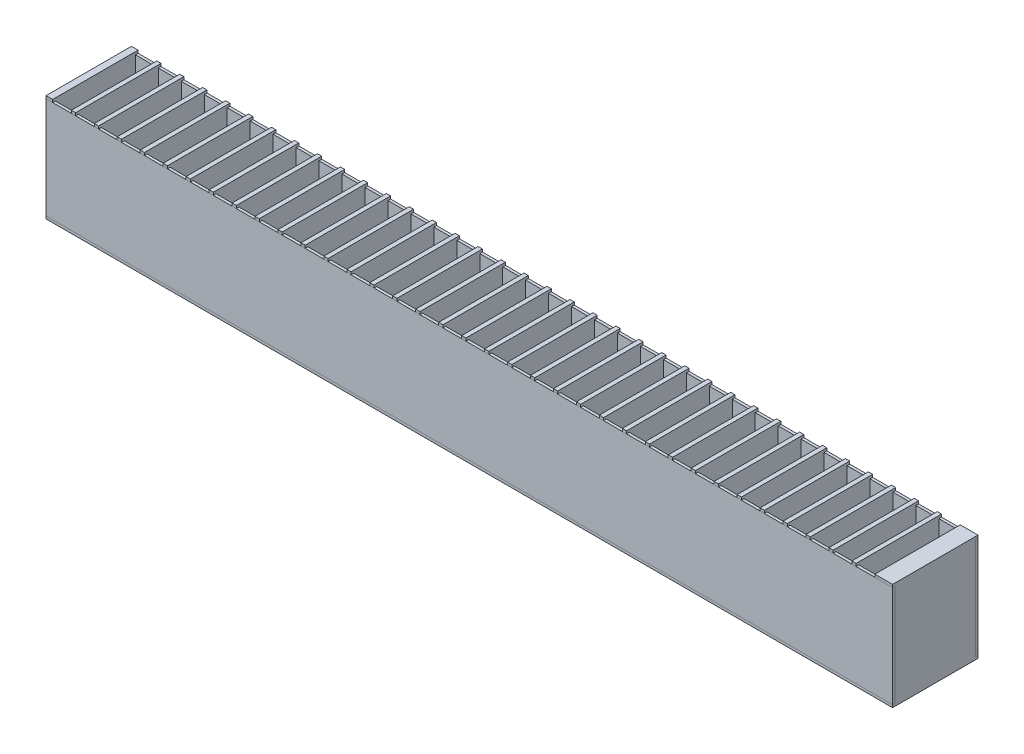
SolidWorks part; units mm, degrees
ref_plane "Front Plane" through (0, 0, 0) normal (0, 0, 1) x (1, 0, 0)
ref_plane "Top Plane" through (0, 0, 0) normal (0, 1, 0) x (1, 0, 0)
ref_plane "Right Plane" through (0, 0, 0) normal (1, 0, 0) x (0, 0, -1)
other "Configuration Table"
sketch "Sketch1" plane through (0, 0, 0) normal (0, 1, 0) x (1, 0, 0)
  line L0 (-0.4, -6) -> (-3.9, -6)
  line L1 (-78.2442, 8) -> (80.3234, 8)
  line L2 (-78.2442, 8) -> (-78.2442, -8)
  line L3 (-78.2442, -8) -> (80.3234, -8)
  line L4 (80.3234, 8) -> (80.3234, -8)
  line L5 (-55, 0) -> (55, 0) construction
  line L6 (0, -55) -> (0, 55) construction
  line L7 (-0.4, 1) -> (-3.9, 1)
  line L8 (-0.4, 1) -> (-0.4, 6)
  line L9 (-0.4, 6) -> (-3.9, 6)
  line L10 (-3.9, 1) -> (-3.9, 6)
  line L11 (-3.9, -1) -> (-3.9, -6)
  line L12 (-0.4, -1) -> (-3.9, -1)
  line L13 (-0.4, -1) -> (-0.4, -6)
  line L14 (3.9, 1) -> (3.9, 6)
  line L15 (3.9, 1) -> (0.4, 1)
  line L16 (0.4, 1) -> (0.4, 6)
  line L17 (3.9, 6) -> (0.4, 6)
  line L18 (3.9, -6) -> (0.4, -6)
  line L19 (0.4, -1) -> (0.4, -6)
  line L20 (3.9, -1) -> (0.4, -1)
  line L21 (3.9, -1) -> (3.9, -6)
  line L22 (8.2, 1) -> (8.2, 6)
  line L23 (8.2, 1) -> (4.7, 1)
  line L24 (4.7, 1) -> (4.7, 6)
  line L25 (8.2, 6) -> (4.7, 6)
  line L26 (8.2, -6) -> (4.7, -6)
  line L27 (4.7, -1) -> (4.7, -6)
  line L28 (8.2, -1) -> (4.7, -1)
  line L29 (8.2, -1) -> (8.2, -6)
  line L30 (12.5, 1) -> (12.5, 6)
  line L31 (12.5, 1) -> (9, 1)
  line L32 (9, 1) -> (9, 6)
  line L33 (12.5, 6) -> (9, 6)
  line L34 (12.5, -6) -> (9, -6)
  line L35 (9, -1) -> (9, -6)
  line L36 (12.5, -1) -> (9, -1)
  line L37 (12.5, -1) -> (12.5, -6)
  line L38 (16.8, 1) -> (16.8, 6)
  line L39 (16.8, 1) -> (13.3, 1)
  line L40 (13.3, 1) -> (13.3, 6)
  line L41 (16.8, 6) -> (13.3, 6)
  line L42 (16.8, -6) -> (13.3, -6)
  line L43 (13.3, -1) -> (13.3, -6)
  line L44 (16.8, -1) -> (13.3, -1)
  line L45 (16.8, -1) -> (16.8, -6)
  line L46 (21.1, 1) -> (21.1, 6)
  line L47 (21.1, 1) -> (17.6, 1)
  line L48 (17.6, 1) -> (17.6, 6)
  line L49 (21.1, 6) -> (17.6, 6)
  line L50 (21.1, -6) -> (17.6, -6)
  line L51 (17.6, -1) -> (17.6, -6)
  line L52 (21.1, -1) -> (17.6, -1)
  line L53 (21.1, -1) -> (21.1, -6)
  line L54 (25.4, 1) -> (25.4, 6)
  line L55 (25.4, 1) -> (21.9, 1)
  line L56 (21.9, 1) -> (21.9, 6)
  line L57 (25.4, 6) -> (21.9, 6)
  line L58 (25.4, -6) -> (21.9, -6)
  line L59 (21.9, -1) -> (21.9, -6)
  line L60 (25.4, -1) -> (21.9, -1)
  line L61 (25.4, -1) -> (25.4, -6)
  line L62 (29.7, 1) -> (29.7, 6)
  line L63 (29.7, 1) -> (26.2, 1)
  line L64 (26.2, 1) -> (26.2, 6)
  line L65 (29.7, 6) -> (26.2, 6)
  line L66 (29.7, -6) -> (26.2, -6)
  line L67 (26.2, -1) -> (26.2, -6)
  line L68 (29.7, -1) -> (26.2, -1)
  line L69 (29.7, -1) -> (29.7, -6)
  line L70 (34, 1) -> (34, 6)
  line L71 (34, 1) -> (30.5, 1)
  line L72 (30.5, 1) -> (30.5, 6)
  line L73 (34, 6) -> (30.5, 6)
  line L74 (34, -6) -> (30.5, -6)
  line L75 (30.5, -1) -> (30.5, -6)
  line L76 (34, -1) -> (30.5, -1)
  line L77 (34, -1) -> (34, -6)
  line L78 (38.3, 1) -> (38.3, 6)
  line L79 (38.3, 1) -> (34.8, 1)
  line L80 (34.8, 1) -> (34.8, 6)
  line L81 (38.3, 6) -> (34.8, 6)
  line L82 (38.3, -6) -> (34.8, -6)
  line L83 (34.8, -1) -> (34.8, -6)
  line L84 (38.3, -1) -> (34.8, -1)
  line L85 (38.3, -1) -> (38.3, -6)
  line L86 (42.6, 1) -> (42.6, 6)
  line L87 (42.6, 1) -> (39.1, 1)
  line L88 (39.1, 1) -> (39.1, 6)
  line L89 (42.6, 6) -> (39.1, 6)
  line L90 (42.6, -6) -> (39.1, -6)
  line L91 (39.1, -1) -> (39.1, -6)
  line L92 (42.6, -1) -> (39.1, -1)
  line L93 (42.6, -1) -> (42.6, -6)
  line L94 (46.9, 1) -> (46.9, 6)
  line L95 (46.9, 1) -> (43.4, 1)
  line L96 (43.4, 1) -> (43.4, 6)
  line L97 (46.9, 6) -> (43.4, 6)
  line L98 (46.9, -6) -> (43.4, -6)
  line L99 (43.4, -1) -> (43.4, -6)
  line L100 (46.9, -1) -> (43.4, -1)
  line L101 (46.9, -1) -> (46.9, -6)
  line L102 (51.2, 1) -> (51.2, 6)
  line L103 (51.2, 1) -> (47.7, 1)
  line L104 (47.7, 1) -> (47.7, 6)
  line L105 (51.2, 6) -> (47.7, 6)
  line L106 (51.2, -6) -> (47.7, -6)
  line L107 (47.7, -1) -> (47.7, -6)
  line L108 (51.2, -1) -> (47.7, -1)
  line L109 (51.2, -1) -> (51.2, -6)
  line L110 (55.5, 1) -> (55.5, 6)
  line L111 (55.5, 1) -> (52, 1)
  line L112 (52, 1) -> (52, 6)
  line L113 (55.5, 6) -> (52, 6)
  line L114 (55.5, -6) -> (52, -6)
  line L115 (52, -1) -> (52, -6)
  line L116 (55.5, -1) -> (52, -1)
  line L117 (55.5, -1) -> (55.5, -6)
  line L118 (59.8, 1) -> (59.8, 6)
  line L119 (59.8, 1) -> (56.3, 1)
  line L120 (56.3, 1) -> (56.3, 6)
  line L121 (59.8, 6) -> (56.3, 6)
  line L122 (59.8, -6) -> (56.3, -6)
  line L123 (56.3, -1) -> (56.3, -6)
  line L124 (59.8, -1) -> (56.3, -1)
  line L125 (59.8, -1) -> (59.8, -6)
  line L126 (64.1, 1) -> (64.1, 6)
  line L127 (64.1, 1) -> (60.6, 1)
  line L128 (60.6, 1) -> (60.6, 6)
  line L129 (64.1, 6) -> (60.6, 6)
  line L130 (64.1, -6) -> (60.6, -6)
  line L131 (60.6, -1) -> (60.6, -6)
  line L132 (64.1, -1) -> (60.6, -1)
  line L133 (64.1, -1) -> (64.1, -6)
  line L134 (68.4, 1) -> (68.4, 6)
  line L135 (68.4, 1) -> (64.9, 1)
  line L136 (64.9, 1) -> (64.9, 6)
  line L137 (68.4, 6) -> (64.9, 6)
  line L138 (68.4, -6) -> (64.9, -6)
  line L139 (64.9, -1) -> (64.9, -6)
  line L140 (68.4, -1) -> (64.9, -1)
  line L141 (68.4, -1) -> (68.4, -6)
  line L142 (72.7, 1) -> (72.7, 6)
  line L143 (72.7, 1) -> (69.2, 1)
  line L144 (69.2, 1) -> (69.2, 6)
  line L145 (72.7, 6) -> (69.2, 6)
  line L146 (72.7, -6) -> (69.2, -6)
  line L147 (69.2, -1) -> (69.2, -6)
  line L148 (72.7, -1) -> (69.2, -1)
  line L149 (72.7, -1) -> (72.7, -6)
  line L150 (-0.4, 1) -> (3.9, 1) construction
  line L151 (-4.7, 1) -> (-4.7, 6)
  line L152 (-4.7, 1) -> (-8.2, 1)
  line L153 (-8.2, 1) -> (-8.2, 6)
  line L154 (-4.7, 6) -> (-8.2, 6)
  line L155 (-4.7, -6) -> (-8.2, -6)
  line L156 (-8.2, -1) -> (-8.2, -6)
  line L157 (-4.7, -1) -> (-8.2, -1)
  line L158 (-4.7, -1) -> (-4.7, -6)
  line L159 (-9, 1) -> (-9, 6)
  line L160 (-9, 1) -> (-12.5, 1)
  line L161 (-12.5, 1) -> (-12.5, 6)
  line L162 (-9, 6) -> (-12.5, 6)
  line L163 (-9, -6) -> (-12.5, -6)
  line L164 (-12.5, -1) -> (-12.5, -6)
  line L165 (-9, -1) -> (-12.5, -1)
  line L166 (-9, -1) -> (-9, -6)
  line L167 (-13.3, 1) -> (-13.3, 6)
  line L168 (-13.3, 1) -> (-16.8, 1)
  line L169 (-16.8, 1) -> (-16.8, 6)
  line L170 (-13.3, 6) -> (-16.8, 6)
  line L171 (-13.3, -6) -> (-16.8, -6)
  line L172 (-16.8, -1) -> (-16.8, -6)
  line L173 (-13.3, -1) -> (-16.8, -1)
  line L174 (-13.3, -1) -> (-13.3, -6)
  line L175 (-17.6, 1) -> (-17.6, 6)
  line L176 (-17.6, 1) -> (-21.1, 1)
  line L177 (-21.1, 1) -> (-21.1, 6)
  line L178 (-17.6, 6) -> (-21.1, 6)
  line L179 (-17.6, -6) -> (-21.1, -6)
  line L180 (-21.1, -1) -> (-21.1, -6)
  line L181 (-17.6, -1) -> (-21.1, -1)
  line L182 (-17.6, -1) -> (-17.6, -6)
  line L183 (-21.9, 1) -> (-21.9, 6)
  line L184 (-21.9, 1) -> (-25.4, 1)
  line L185 (-25.4, 1) -> (-25.4, 6)
  line L186 (-21.9, 6) -> (-25.4, 6)
  line L187 (-21.9, -6) -> (-25.4, -6)
  line L188 (-25.4, -1) -> (-25.4, -6)
  line L189 (-21.9, -1) -> (-25.4, -1)
  line L190 (-21.9, -1) -> (-21.9, -6)
  line L191 (-26.2, 1) -> (-26.2, 6)
  line L192 (-26.2, 1) -> (-29.7, 1)
  line L193 (-29.7, 1) -> (-29.7, 6)
  line L194 (-26.2, 6) -> (-29.7, 6)
  line L195 (-26.2, -6) -> (-29.7, -6)
  line L196 (-29.7, -1) -> (-29.7, -6)
  line L197 (-26.2, -1) -> (-29.7, -1)
  line L198 (-26.2, -1) -> (-26.2, -6)
  line L199 (-30.5, 1) -> (-30.5, 6)
  line L200 (-30.5, 1) -> (-34, 1)
  line L201 (-34, 1) -> (-34, 6)
  line L202 (-30.5, 6) -> (-34, 6)
  line L203 (-30.5, -6) -> (-34, -6)
  line L204 (-34, -1) -> (-34, -6)
  line L205 (-30.5, -1) -> (-34, -1)
  line L206 (-30.5, -1) -> (-30.5, -6)
  line L207 (-34.8, 1) -> (-34.8, 6)
  line L208 (-34.8, 1) -> (-38.3, 1)
  line L209 (-38.3, 1) -> (-38.3, 6)
  line L210 (-34.8, 6) -> (-38.3, 6)
  line L211 (-34.8, -6) -> (-38.3, -6)
  line L212 (-38.3, -1) -> (-38.3, -6)
  line L213 (-34.8, -1) -> (-38.3, -1)
  line L214 (-34.8, -1) -> (-34.8, -6)
  line L215 (-39.1, 1) -> (-39.1, 6)
  line L216 (-39.1, 1) -> (-42.6, 1)
  line L217 (-42.6, 1) -> (-42.6, 6)
  line L218 (-39.1, 6) -> (-42.6, 6)
  line L219 (-39.1, -6) -> (-42.6, -6)
  line L220 (-42.6, -1) -> (-42.6, -6)
  line L221 (-39.1, -1) -> (-42.6, -1)
  line L222 (-39.1, -1) -> (-39.1, -6)
  line L223 (-43.4, 1) -> (-43.4, 6)
  line L224 (-43.4, 1) -> (-46.9, 1)
  line L225 (-46.9, 1) -> (-46.9, 6)
  line L226 (-43.4, 6) -> (-46.9, 6)
  line L227 (-43.4, -6) -> (-46.9, -6)
  line L228 (-46.9, -1) -> (-46.9, -6)
  line L229 (-43.4, -1) -> (-46.9, -1)
  line L230 (-43.4, -1) -> (-43.4, -6)
  line L231 (-47.7, 1) -> (-47.7, 6)
  line L232 (-47.7, 1) -> (-51.2, 1)
  line L233 (-51.2, 1) -> (-51.2, 6)
  line L234 (-47.7, 6) -> (-51.2, 6)
  line L235 (-47.7, -6) -> (-51.2, -6)
  line L236 (-51.2, -1) -> (-51.2, -6)
  line L237 (-47.7, -1) -> (-51.2, -1)
  line L238 (-47.7, -1) -> (-47.7, -6)
  line L239 (-52, 1) -> (-52, 6)
  line L240 (-52, 1) -> (-55.5, 1)
  line L241 (-55.5, 1) -> (-55.5, 6)
  line L242 (-52, 6) -> (-55.5, 6)
  line L243 (-52, -6) -> (-55.5, -6)
  line L244 (-55.5, -1) -> (-55.5, -6)
  line L245 (-52, -1) -> (-55.5, -1)
  line L246 (-52, -1) -> (-52, -6)
  line L247 (-56.3, 1) -> (-56.3, 6)
  line L248 (-56.3, 1) -> (-59.8, 1)
  line L249 (-59.8, 1) -> (-59.8, 6)
  line L250 (-56.3, 6) -> (-59.8, 6)
  line L251 (-56.3, -6) -> (-59.8, -6)
  line L252 (-59.8, -1) -> (-59.8, -6)
  line L253 (-56.3, -1) -> (-59.8, -1)
  line L254 (-56.3, -1) -> (-56.3, -6)
  line L255 (-60.6, 1) -> (-60.6, 6)
  line L256 (-60.6, 1) -> (-64.1, 1)
  line L257 (-64.1, 1) -> (-64.1, 6)
  line L258 (-60.6, 6) -> (-64.1, 6)
  line L259 (-60.6, -6) -> (-64.1, -6)
  line L260 (-64.1, -1) -> (-64.1, -6)
  line L261 (-60.6, -1) -> (-64.1, -1)
  line L262 (-60.6, -1) -> (-60.6, -6)
  line L263 (-64.9, 1) -> (-64.9, 6)
  line L264 (-64.9, 1) -> (-68.4, 1)
  line L265 (-68.4, 1) -> (-68.4, 6)
  line L266 (-64.9, 6) -> (-68.4, 6)
  line L267 (-64.9, -6) -> (-68.4, -6)
  line L268 (-68.4, -1) -> (-68.4, -6)
  line L269 (-64.9, -1) -> (-68.4, -1)
  line L270 (-64.9, -1) -> (-64.9, -6)
  line L271 (-69.2, 1) -> (-69.2, 6)
  line L272 (-69.2, 1) -> (-72.7, 1)
  line L273 (-72.7, 1) -> (-72.7, 6)
  line L274 (-69.2, 6) -> (-72.7, 6)
  line L275 (-69.2, -6) -> (-72.7, -6)
  line L276 (-72.7, -1) -> (-72.7, -6)
  line L277 (-69.2, -1) -> (-72.7, -1)
  line L278 (-69.2, -1) -> (-69.2, -6)
  line L279 (-0.4, 1) -> (-4.7, 1) construction
  line L280 (-73.5, 1) -> (-73.5, 6)
  line L281 (-73.5, 1) -> (-77, 1)
  line L282 (-77, 1) -> (-77, 6)
  line L283 (-73.5, 6) -> (-77, 6)
  line L284 (-73.5, -6) -> (-77, -6)
  line L285 (-77, -1) -> (-77, -6)
  line L286 (-73.5, -1) -> (-77, -1)
  line L287 (-73.5, -1) -> (-73.5, -6)
  line L288 (77, 1) -> (77, 6)
  line L289 (77, 1) -> (73.5, 1)
  line L290 (73.5, 1) -> (73.5, 6)
  line L291 (77, 6) -> (73.5, 6)
  line L292 (77, -6) -> (73.5, -6)
  line L293 (73.5, -1) -> (73.5, -6)
  line L294 (77, -1) -> (73.5, -1)
  line L295 (77, -1) -> (77, -6)
  dimension "D1" = 8
  dimension "D2" = 8
  dimension "D3" = 0.4
  dimension "D4" = 1
  dimension "D5" = 3.5
  dimension "D7" = 4.3
  dimension "D9" = 4.3
  dimension "D10" = 5
  dimension "D6" = 19
  dimension "D8" = 18
extrude "Boss-Extrude1" add sketch "Sketch1" along normal mid plane 20
sketch "Sketch4" plane through (0, 0, 8) normal (0, 0, 1) x (1, 0, 0)
  line L0 (-78.2442, 10) -> (80.3234, 10) construction
  line L1 (-3.9, 10) -> (-0.4, 10)
  line L2 (-3.9, 10) -> (-3.9, -9.5)
  line L3 (-3.9, -9.5) -> (-0.4, -9.5)
  line L4 (-0.4, 10) -> (-0.4, -9.5)
  line L5 (-78.2442, -10) -> (80.3234, -10) construction
  line L6 (0, -8.8) -> (0, 8.8) construction
  line L7 (0.4, 10) -> (0.4, -9.5)
  line L8 (0.4, 10) -> (3.9, 10)
  line L9 (3.9, 10) -> (3.9, -9.5)
  line L10 (0.4, -9.5) -> (3.9, -9.5)
  line L11 (4.7, 10) -> (4.7, -9.5)
  line L12 (4.7, 10) -> (8.2, 10)
  line L13 (8.2, 10) -> (8.2, -9.5)
  line L14 (4.7, -9.5) -> (8.2, -9.5)
  line L15 (9, 10) -> (9, -9.5)
  line L16 (9, 10) -> (12.5, 10)
  line L17 (12.5, 10) -> (12.5, -9.5)
  line L18 (9, -9.5) -> (12.5, -9.5)
  line L19 (13.3, 10) -> (13.3, -9.5)
  line L20 (13.3, 10) -> (16.8, 10)
  line L21 (16.8, 10) -> (16.8, -9.5)
  line L22 (13.3, -9.5) -> (16.8, -9.5)
  line L23 (17.6, 10) -> (17.6, -9.5)
  line L24 (17.6, 10) -> (21.1, 10)
  line L25 (21.1, 10) -> (21.1, -9.5)
  line L26 (17.6, -9.5) -> (21.1, -9.5)
  line L27 (21.9, 10) -> (21.9, -9.5)
  line L28 (21.9, 10) -> (25.4, 10)
  line L29 (25.4, 10) -> (25.4, -9.5)
  line L30 (21.9, -9.5) -> (25.4, -9.5)
  line L31 (26.2, 10) -> (26.2, -9.5)
  line L32 (26.2, 10) -> (29.7, 10)
  line L33 (29.7, 10) -> (29.7, -9.5)
  line L34 (26.2, -9.5) -> (29.7, -9.5)
  line L35 (30.5, 10) -> (30.5, -9.5)
  line L36 (30.5, 10) -> (34, 10)
  line L37 (34, 10) -> (34, -9.5)
  line L38 (30.5, -9.5) -> (34, -9.5)
  line L39 (34.8, 10) -> (34.8, -9.5)
  line L40 (34.8, 10) -> (38.3, 10)
  line L41 (38.3, 10) -> (38.3, -9.5)
  line L42 (34.8, -9.5) -> (38.3, -9.5)
  line L43 (39.1, 10) -> (39.1, -9.5)
  line L44 (39.1, 10) -> (42.6, 10)
  line L45 (42.6, 10) -> (42.6, -9.5)
  line L46 (39.1, -9.5) -> (42.6, -9.5)
  line L47 (43.4, 10) -> (43.4, -9.5)
  line L48 (43.4, 10) -> (46.9, 10)
  line L49 (46.9, 10) -> (46.9, -9.5)
  line L50 (43.4, -9.5) -> (46.9, -9.5)
  line L51 (47.7, 10) -> (47.7, -9.5)
  line L52 (47.7, 10) -> (51.2, 10)
  line L53 (51.2, 10) -> (51.2, -9.5)
  line L54 (47.7, -9.5) -> (51.2, -9.5)
  line L55 (52, 10) -> (52, -9.5)
  line L56 (52, 10) -> (55.5, 10)
  line L57 (55.5, 10) -> (55.5, -9.5)
  line L58 (52, -9.5) -> (55.5, -9.5)
  line L59 (56.3, 10) -> (56.3, -9.5)
  line L60 (56.3, 10) -> (59.8, 10)
  line L61 (59.8, 10) -> (59.8, -9.5)
  line L62 (56.3, -9.5) -> (59.8, -9.5)
  line L63 (60.6, 10) -> (60.6, -9.5)
  line L64 (60.6, 10) -> (64.1, 10)
  line L65 (64.1, 10) -> (64.1, -9.5)
  line L66 (60.6, -9.5) -> (64.1, -9.5)
  line L67 (64.9, 10) -> (64.9, -9.5)
  line L68 (64.9, 10) -> (68.4, 10)
  line L69 (68.4, 10) -> (68.4, -9.5)
  line L70 (64.9, -9.5) -> (68.4, -9.5)
  line L71 (69.2, 10) -> (69.2, -9.5)
  line L72 (69.2, 10) -> (72.7, 10)
  line L73 (72.7, 10) -> (72.7, -9.5)
  line L74 (69.2, -9.5) -> (72.7, -9.5)
  line L75 (73.5, 10) -> (73.5, -9.5)
  line L76 (73.5, 10) -> (77, 10)
  line L77 (77, 10) -> (77, -9.5)
  line L78 (73.5, -9.5) -> (77, -9.5)
  line L79 (-3.9, 10) -> (0.4, 10) construction
  line L80 (-8.2, 10) -> (-8.2, -9.5)
  line L81 (-8.2, 10) -> (-4.7, 10)
  line L82 (-4.7, 10) -> (-4.7, -9.5)
  line L83 (-8.2, -9.5) -> (-4.7, -9.5)
  line L84 (-12.5, 10) -> (-12.5, -9.5)
  line L85 (-12.5, 10) -> (-9, 10)
  line L86 (-9, 10) -> (-9, -9.5)
  line L87 (-12.5, -9.5) -> (-9, -9.5)
  line L88 (-16.8, 10) -> (-16.8, -9.5)
  line L89 (-16.8, 10) -> (-13.3, 10)
  line L90 (-13.3, 10) -> (-13.3, -9.5)
  line L91 (-16.8, -9.5) -> (-13.3, -9.5)
  line L92 (-21.1, 10) -> (-21.1, -9.5)
  line L93 (-21.1, 10) -> (-17.6, 10)
  line L94 (-17.6, 10) -> (-17.6, -9.5)
  line L95 (-21.1, -9.5) -> (-17.6, -9.5)
  line L96 (-25.4, 10) -> (-25.4, -9.5)
  line L97 (-25.4, 10) -> (-21.9, 10)
  line L98 (-21.9, 10) -> (-21.9, -9.5)
  line L99 (-25.4, -9.5) -> (-21.9, -9.5)
  line L100 (-29.7, 10) -> (-29.7, -9.5)
  line L101 (-29.7, 10) -> (-26.2, 10)
  line L102 (-26.2, 10) -> (-26.2, -9.5)
  line L103 (-29.7, -9.5) -> (-26.2, -9.5)
  line L104 (-34, 10) -> (-34, -9.5)
  line L105 (-34, 10) -> (-30.5, 10)
  line L106 (-30.5, 10) -> (-30.5, -9.5)
  line L107 (-34, -9.5) -> (-30.5, -9.5)
  line L108 (-38.3, 10) -> (-38.3, -9.5)
  line L109 (-38.3, 10) -> (-34.8, 10)
  line L110 (-34.8, 10) -> (-34.8, -9.5)
  line L111 (-38.3, -9.5) -> (-34.8, -9.5)
  line L112 (-42.6, 10) -> (-42.6, -9.5)
  line L113 (-42.6, 10) -> (-39.1, 10)
  line L114 (-39.1, 10) -> (-39.1, -9.5)
  line L115 (-42.6, -9.5) -> (-39.1, -9.5)
  line L116 (-46.9, 10) -> (-46.9, -9.5)
  line L117 (-46.9, 10) -> (-43.4, 10)
  line L118 (-43.4, 10) -> (-43.4, -9.5)
  line L119 (-46.9, -9.5) -> (-43.4, -9.5)
  line L120 (-51.2, 10) -> (-51.2, -9.5)
  line L121 (-51.2, 10) -> (-47.7, 10)
  line L122 (-47.7, 10) -> (-47.7, -9.5)
  line L123 (-51.2, -9.5) -> (-47.7, -9.5)
  line L124 (-55.5, 10) -> (-55.5, -9.5)
  line L125 (-55.5, 10) -> (-52, 10)
  line L126 (-52, 10) -> (-52, -9.5)
  line L127 (-55.5, -9.5) -> (-52, -9.5)
  line L128 (-59.8, 10) -> (-59.8, -9.5)
  line L129 (-59.8, 10) -> (-56.3, 10)
  line L130 (-56.3, 10) -> (-56.3, -9.5)
  line L131 (-59.8, -9.5) -> (-56.3, -9.5)
  line L132 (-64.1, 10) -> (-64.1, -9.5)
  line L133 (-64.1, 10) -> (-60.6, 10)
  line L134 (-60.6, 10) -> (-60.6, -9.5)
  line L135 (-64.1, -9.5) -> (-60.6, -9.5)
  line L136 (-68.4, 10) -> (-68.4, -9.5)
  line L137 (-68.4, 10) -> (-64.9, 10)
  line L138 (-64.9, 10) -> (-64.9, -9.5)
  line L139 (-68.4, -9.5) -> (-64.9, -9.5)
  line L140 (-72.7, 10) -> (-72.7, -9.5)
  line L141 (-72.7, 10) -> (-69.2, 10)
  line L142 (-69.2, 10) -> (-69.2, -9.5)
  line L143 (-72.7, -9.5) -> (-69.2, -9.5)
  line L144 (-77, 10) -> (-77, -9.5)
  line L145 (-77, 10) -> (-73.5, 10)
  line L146 (-73.5, 10) -> (-73.5, -9.5)
  line L147 (-77, -9.5) -> (-73.5, -9.5)
  line L148 (-3.9, 10) -> (-8.2, 10) construction
  dimension "D1" = 0.5
  dimension "D2" = 0.4
  dimension "D3" = 3.5
  dimension "D5" = 4.3
  dimension "D7" = 4.3
  dimension "D4" = 19
  dimension "D6" = 18
extrude "Cut-Extrude2" cut sketch "Sketch4" against normal up to surface (9 mm away)
mirror "Mirror1" about plane through (0, 0, 0) normal (0, 0, 1) of "Cut-Extrude2"
sketch "Sketch2" plane through (80.3234, 0, 0) normal (1, 0, 0) x (0, 0, -1)
  line L0 (-8, 10) -> (-8, -10) construction
  line L1 (-8, 9.5) -> (-7.5, 9.5)
  line L2 (-8, 9.5) -> (-8, -9.5)
  line L3 (-8, -9.5) -> (-7.5, -9.5)
  line L4 (-7.5, 9.5) -> (-7.5, -9.5)
  line L6 (-8, 10) -> (8, 10) construction
  line L7 (-8, -10) -> (8, -10) construction
  line L8 (0, 11) -> (0, -11) construction
  line L9 (8, -9.5) -> (7.5, -9.5)
  line L10 (7.5, 9.5) -> (7.5, -9.5)
  line L11 (8, 9.5) -> (7.5, 9.5)
  line L12 (8, 9.5) -> (8, -9.5)
  dimension "D1" = 0.5
  dimension "D2" = 0.5
  dimension "D3" = 0.5
extrude "Cut-Extrude1" cut sketch "Sketch2" against normal up to surface (158.5676 mm away) up to face at (-78.2442, 0, 0)
sketch "Sketch3" plane through (80.3234, 0, 0) normal (1, 0, 0) x (0, 0, -1)
  line L1 (-8, 9.5) -> (-7.5, 9.5)
  line L2 (-8, 9.5) -> (-8, -9.5)
  line L3 (-8, -9.5) -> (-7.5, -9.5)
  line L4 (-7.5, 9.5) -> (-7.5, -9.5)
  line L5 (7.5, 9.5) -> (8, 9.5)
  line L6 (7.5, 9.5) -> (7.5, -9.5)
  line L7 (7.5, -9.5) -> (8, -9.5)
  line L8 (8, 9.5) -> (8, -9.5)
extrude "Boss-Extrude2" add sketch "Sketch3" against normal up to surface (158.5676 mm away) separate body up to face at (-78.2442, 0, 0)
